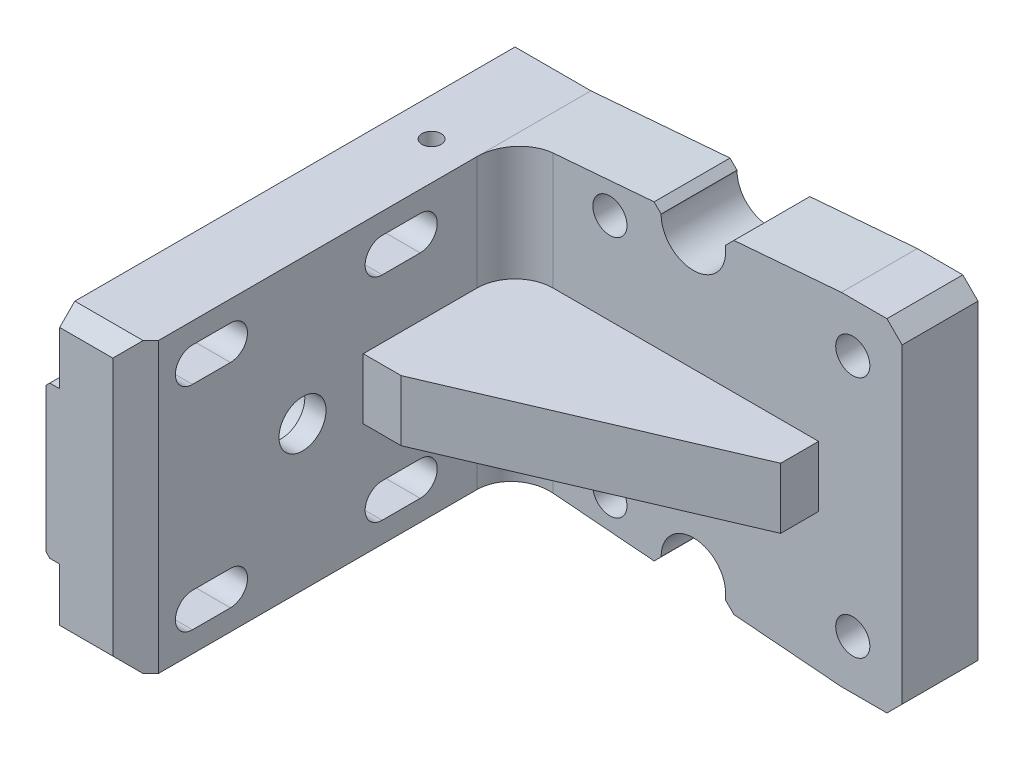
SolidWorks part; units mm, degrees
ref_plane "Front Plane" through (0, 0, 0) normal (0, 0, 1) x (1, 0, 0)
ref_plane "Top Plane" through (0, 0, 0) normal (0, 1, 0) x (1, 0, 0)
ref_plane "Right Plane" through (0, 0, 0) normal (1, 0, 0) x (0, 0, -1)
sketch "Sketch1" plane through (0, 0, 0) normal (0, 0, 1) x (1, 0, 0)
  line L1 (-30.5, -22.5) -> (30.5, -22.5)
  line L2 (-30.5, -22.5) -> (-30.5, 22.5)
  line L3 (-30.5, 22.5) -> (30.5, 22.5)
  line L4 (30.5, -22.5) -> (30.5, 22.5)
  line L5 (-30.5, -22.5) -> (30.5, 22.5) construction
  line L6 (-30.5, 22.5) -> (30.5, -22.5) construction
  point P0 (0, 0)
  dimension "D1" = 45
  dimension "D2" = 61
extrude "Boss-Extrude1" add sketch "Sketch1" along normal blind 10
sketch "Sketch2" plane through (0, 0, 10) normal (0, 0, 1) x (1, 0, 0)
  line L0 (-30.5, -22.5) -> (30.5, -22.5) construction
  line L1 (-30.5, 22.5) -> (-20.5, 22.5)
  line L2 (-30.5, 22.5) -> (-30.5, -22.5)
  line L3 (-30.5, -22.5) -> (-20.5, -22.5)
  line L4 (-20.5, 22.5) -> (-20.5, -22.5)
  dimension "D1" = 10
extrude "Boss-Extrude2" add sketch "Sketch2" along normal blind 50
sketch "Sketch4" plane through (-30.5, 0, 0) normal (-1, 0, 0) x (0, 0, 1)
  line L0 (60, 22.5) -> (60, -22.5) construction
  line L1 (60, 10) -> (0, 10)
  line L2 (60, 10) -> (60, -10)
  line L3 (60, -10) -> (0, -10)
  line L4 (0, 10) -> (0, -10)
  line L5 (0, 22.5) -> (0, -22.5) construction
  line L6 (0, 0) -> (88.2751, 0) construction
  dimension "D1" = 20
sketch "Sketch5" plane through (-20.5, 0, 0) normal (1, 0, 0) x (0, 0, -1)
  line L0 (-52.5, -14) -> (-47.5, -14) construction
  line L1 (-52.5, -11.75) -> (-47.5, -11.75)
  line L2 (-52.5, -16.25) -> (-47.5, -16.25)
  line L4 (-60, -22.5) -> (-60, 22.5) construction
  line L5 (-10, -22.5) -> (0, -22.5) construction
  arc A0 (-52.5, -11.75) -> (-52.5, -16.25) centre (-52.5, -14) ccw
  arc A1 (-47.5, -16.25) -> (-47.5, -11.75) centre (-47.5, -14) ccw
  point P2 (-50, -14)
  dimension "D1" = 4.5
  dimension "D2" = 5
  dimension "D3" = 8.5
  dimension "D4" = 10
extrude "Cut-Extrude3" cut sketch "Sketch5" against normal through all
sketch "Sketch6" plane through (0, 0, 10) normal (0, 0, 1) x (1, 0, 0)
  line L0 (-20.5, 0) -> (41.1665, 0) construction
  line L1 (-20.5, -22.5) -> (-20.5, 22.5) construction
  line L3 (-20.5, 4) -> (19.5, 4)
  line L4 (-20.5, 4) -> (-20.5, -4)
  line L5 (-20.5, -4) -> (19.5, -4)
  line L6 (19.5, 4) -> (19.5, -4)
  dimension "D1" = 8
  dimension "D2" = 40
extrude "Boss-Extrude3" add sketch "Sketch6" along normal blind 20
sketch "Sketch7" plane through (0, -4, 0) normal (0, -1, 0) x (1, 0, 0)
  line L0 (19.5, 30) -> (-15.5, 30)
  line L1 (-20.5, 30) -> (19.5, 30) construction
  line L2 (-15.5, 30) -> (19.5, 15)
  line L3 (19.5, 30) -> (19.5, 10) construction
  line L4 (19.5, 15) -> (19.5, 30)
  line L5 (-20.5, 60) -> (-20.5, 10) construction
  line L7 (-20.5, 10) -> (30.5, 10) construction
  dimension "D1" = 5
  dimension "D2" = 5
extrude "Cut-Extrude4" cut sketch "Sketch7" against normal through all
fillet "Fillet1" radius 5 2 edges
sketch "Sketch8" plane through (0, 0, 60) normal (0, 0, 1) x (1, 0, 0)
  line L0 (-30.5, 22.5) -> (22.5, 22.5)
  line L1 (30.5, 22.5) -> (-15.5, 22.5) construction
  line L2 (-20.5, 19) -> (22.5, 22.5)
  line L3 (-20.5, -19) -> (22.5, -22.5)
  line L4 (-30.5, 19) -> (-30.5, 22.5)
  line L5 (-30.5, -22.5) -> (-30.5, -19)
  line L6 (-30.5, 22.5) -> (-30.5, -22.5) construction
  line L8 (-15.5, -22.5) -> (30.5, -22.5) construction
  line L9 (22.5, -22.5) -> (-30.5, -22.5)
  line L10 (30.5, -22.5) -> (30.5, 22.5) construction
  line L11 (-30.5, 19) -> (-20.5, 19)
  line L12 (-20.5, -22.5) -> (-20.5, 22.5) construction
  line L13 (-30.5, -19) -> (-20.5, -19)
  dimension "D1" = 8
  dimension "D2" = 3.5
extrude "Cut-Extrude5" cut sketch "Sketch8" against normal through all
pattern_linear "LPattern2" count 2 spacing 28 along (0, 1, 0) count 2 spacing 25 along (0, 0, -1) of "Cut-Extrude3"
sketch "Sketch9" plane through (0, 0, 0) normal (0, 0, -1) x (-1, 0, 0)
  line L0 (8.75, 0) -> (7.25, 0) construction
  line L1 (8.75, -3) -> (7.25, -3)
  line L2 (8.75, 3) -> (7.25, 3)
  line L3 (-30.5, 0) -> (37.9763, 0) construction
  line L4 (-30.5, -22.5) -> (-30.5, 22.5) construction
  circle A0 centre (-25, 0) radius 3
  arc A1 (8.75, -3) -> (8.75, 3) centre (8.75, 0) ccw
  arc A2 (7.25, 3) -> (7.25, -3) centre (7.25, 0) ccw
  point P5 (8, 0)
  dimension "D1" = 6
  dimension "D2" = 1.5
  dimension "D3" = 33
  dimension "D4" = 5.5
extrude "Cut-Extrude6" cut sketch "Sketch9" against normal blind 5
sketch "Sketch10" plane through (0, 0, 0) normal (0, 0, -1) x (-1, 0, 0)
  line L0 (-30.5, 0) -> (35.1037, 0) construction
  line L1 (-30.5, -22.5) -> (-30.5, 22.5) construction
  line L2 (8, -16) -> (-24, -16) construction
  line L3 (-24, -16) -> (-24, 16) construction
  line L4 (-24, 16) -> (8, 16) construction
  line L5 (8, 16) -> (8, -16) construction
  circle A0 centre (8, -16) radius 2.25
  circle A1 centre (-24, -16) radius 2.25
  circle A2 centre (-24, 16) radius 2.25
  circle A3 centre (8, 16) radius 2.25
  dimension "D4" = 4.5
  dimension "D1" = 32
  dimension "D2" = 32
  dimension "D3" = 6.5
extrude "Cut-Extrude7" cut sketch "Sketch10" against normal through all
chamfer "Chamfer1" distance 2 angle 45 4 edges at (30.5, -22.5, 5) (30.5, 22.5, 5) (-25.5, -19, 60) (-25.5, 19, 60)
hole_wizard "M3 Tapped Hole1" positions "Sketch14" profile "Sketch13" tap size "M3" standard "Gb"
sketch "Sketch14" plane through (0, 19, 0) normal (0, 1, 0) x (1, 0, 0)
  line L0 (-25.5, -55) -> (-25.5, 0) construction
  line L2 (-30.5, 0) -> (-20.5, 0) construction
  point P0 (-25.5, -16)
  dimension "D1" = 16
sketch "Sketch13" plane through (-25.5, 19, 16) normal (1, 0, 0) x (0, 0, 1)
  line L0 (0, 0) -> (0, 8.2511)
  line L1 (0, 8.2511) -> (1.25, 7.5)
  line L2 (1.25, 7.5) -> (1.25, 0)
  line L5 (1.25, 0) -> (0, 0)
  line L10 (0, 8.2511) -> (-1.25, 7.5) construction
  line L11 (0, -6.35) -> (0, 107.95) construction
  dimension "螺纹孔钻头直径" = 2.5
  dimension "螺纹孔钻头深度" = 7.5
  dimension "导头角度" = 118
cosmetic thread "Hole thread 1" parameters "D1"=6, "D2"=3
mirror "Mirror1" about plane through (0, 0, 0) normal (0, 1, 0) of "M3 Tapped Hole1"
extrude "Boss-Extrude4" add sketch "Sketch4" along normal blind 1.8
chamfer "Chamfer2" distance 0.5 angle 45 2 edges at (-32.3, 10, 30) (-32.3, -10, 30)
sketch "Sketch15" plane through (-20.5, 0, 0) normal (1, 0, 0) x (0, 0, -1)
  line L0 (-60, 0) -> (-38, 0) construction
  line L1 (-60, -17) -> (-60, 17) construction
  circle A0 centre (-38, 0) radius 3.1
  dimension "D1" = 6.2
  dimension "D2" = 22
extrude "Cut-Extrude8" cut sketch "Sketch15" against normal through all
sketch "Sketch16" plane through (-32.3, 0, 0) normal (-1, 0, 0) x (0, 0, 1)
  circle A0 centre (38, 0) radius 4.05
  dimension "D1" = 8.1
extrude "Cut-Extrude9" cut sketch "Sketch16" against normal blind 9
sketch "Sketch17" plane through (0, 0, 10) normal (0, 0, 1) x (1, 0, 0)
  line L0 (3, -19.5) -> (3, -28.9438) construction
  line L1 (7.25, -19.5) -> (7.25, -28.9438)
  line L2 (-1.25, -19.5) -> (-1.25, -28.9438)
  line L3 (3, 19.5) -> (3, 28.9438) construction
  line L4 (-1.25, 19.5) -> (-1.25, 28.9438)
  line L5 (7.25, 19.5) -> (7.25, 28.9438)
  line L6 (30.5, -20.5) -> (30.5, 20.5) construction
  line L7 (0, 0) -> (34.1693, 0) construction
  arc A0 (7.25, -19.5) -> (-1.25, -19.5) centre (3, -19.5) ccw
  arc A1 (-1.25, -28.9438) -> (7.25, -28.9438) centre (3, -28.9438) ccw
  arc A2 (-1.25, 19.5) -> (7.25, 19.5) centre (3, 19.5) ccw
  arc A3 (7.25, 28.9438) -> (-1.25, 28.9438) centre (3, 28.9438) ccw
  point P2 (3, -24.2219)
  point P7 (3, 24.2219)
  dimension "D1" = 8.5
  dimension "D2" = 27.5
  dimension "D3" = 39
extrude "Cut-Extrude10" cut sketch "Sketch17" against normal blind 10
chamfer "Chamfer3" distance 1 angle 45 4 edges at (7.25, -21.2587, 5) (-1.25, -20.5669, 5) (-1.25, 20.5669, 5) (7.25, 21.2587, 5)
chamfer "Chamfer4" distance 3 angle 45 1 edges at (-20.5, 0, 60)
